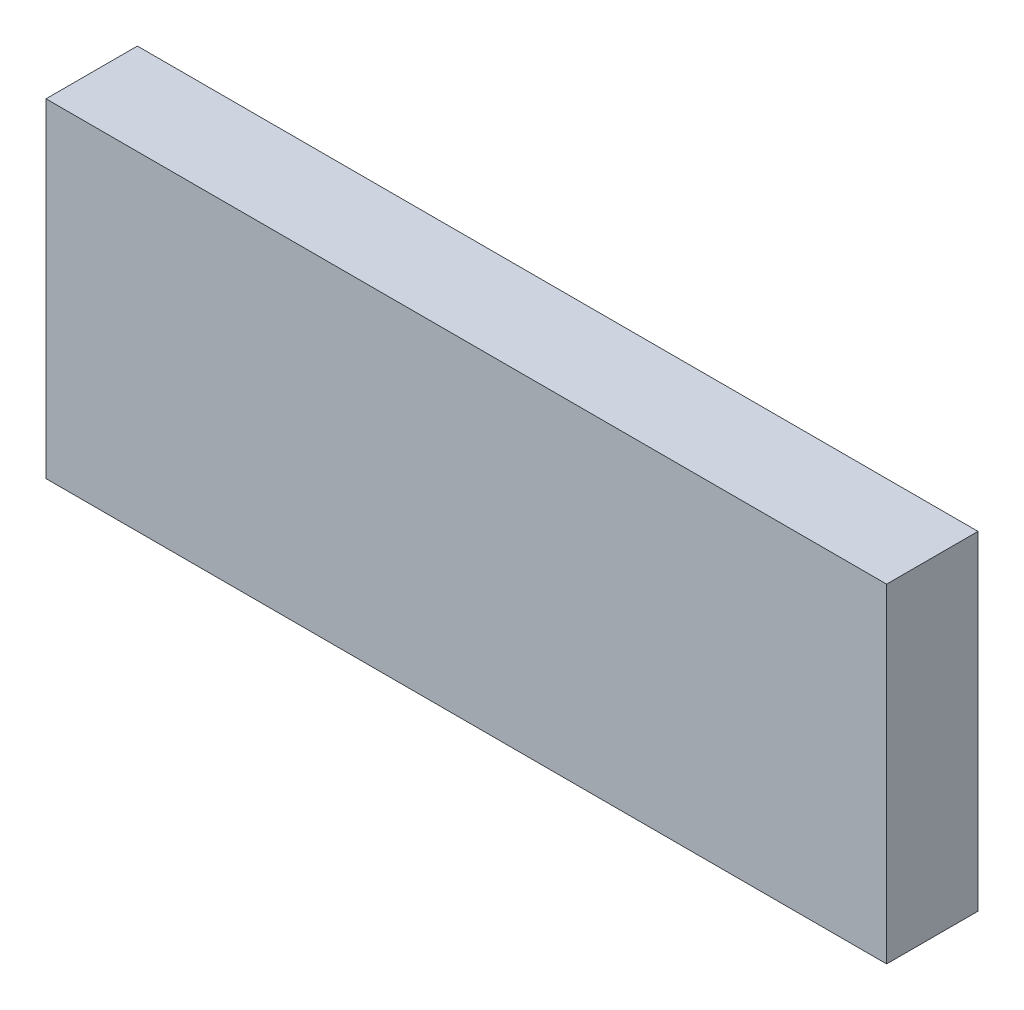
from build123d import *

# Parameters (mm, degrees)
SKETCH1_W           = 230
SKETCH1_H           = 90
BOSS_EXTRUDE1_DEPTH = 25


with BuildPart() as part:
    # Sketch1 → Boss-Extrude1 (new body)
    with BuildSketch(Plane.XY):
        with Locations((-115, 45)):
            Rectangle(SKETCH1_W, SKETCH1_H)
    extrude(amount=BOSS_EXTRUDE1_DEPTH)


solid = part.part
